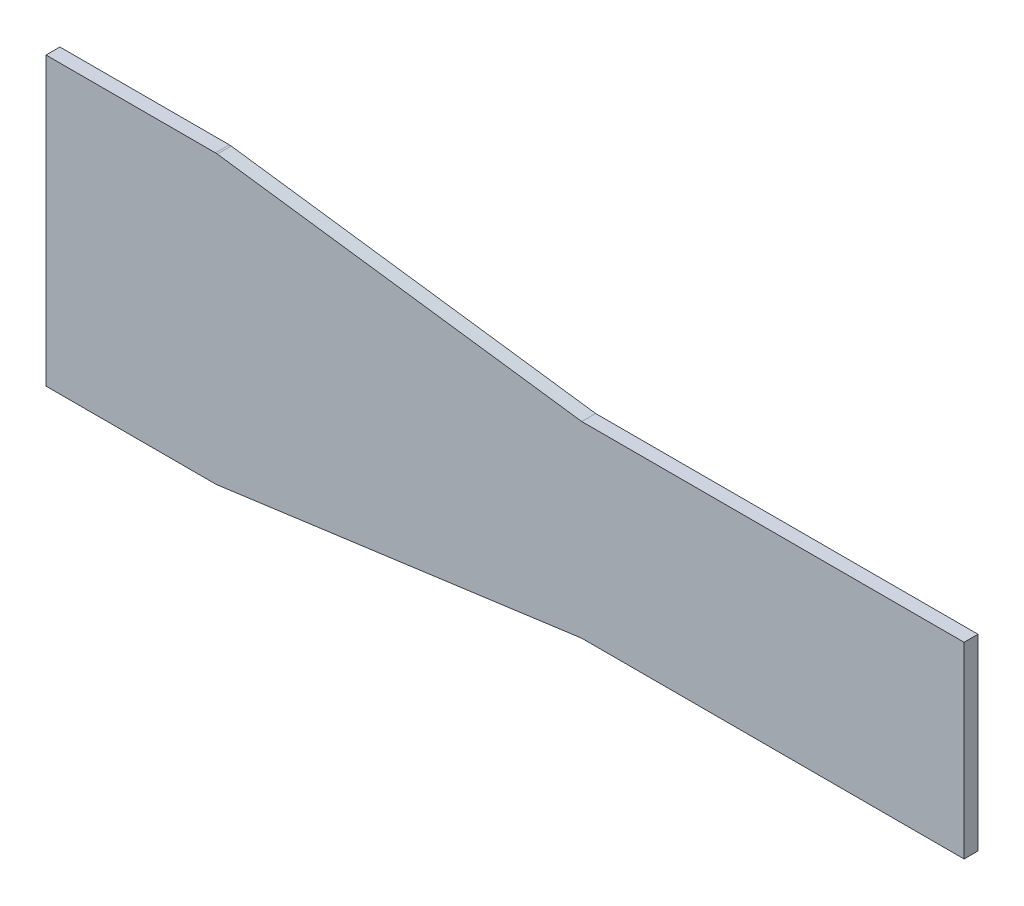
from build123d import *

# Parameters (mm, degrees)
BOSS_EXTRUDE1_DEPTH = 16


with BuildPart() as part:
    # Sketch1 → Boss-Extrude1 (new body)
    with BuildSketch(Plane.XY):
        with BuildLine():
            Line((0, 165), (194.920512906, 165))
            ThreePointArc((194.920512906, 165), (195.997551485, 164.963708463), (197.06970414, 164.854998488))
            Line((197.06970414, 164.854998488), (616.5, 108))
            Line((616.5, 108), (1056.5, 108))
            Line((1056.5, 108), (1056.5, -108))
            Line((1056.5, -108), (616.5, -108))
            Line((616.5, -108), (197.06970414, -164.854998488))
            ThreePointArc((197.06970414, -164.854998488), (195.997551485, -164.963708463), (194.920512906, -165))
            Line((194.920512906, -165), (0, -165))
            Line((0, -165), (0, 165))
        make_face()
    extrude(amount=BOSS_EXTRUDE1_DEPTH)


solid = part.part
